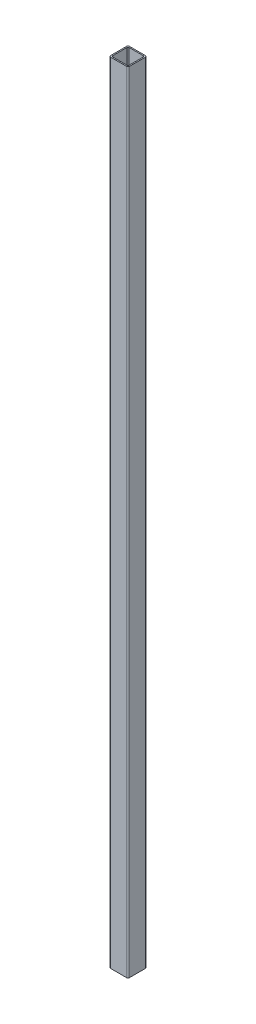
from build123d import *

# Parameters (mm, degrees)
BOSS_EXTRUDE1_DEPTH = 2100


with BuildPart() as part:
    # Sketch2 → Boss-Extrude1 (new, symmetric)
    with BuildSketch(Plane(origin=(0, 0, 0), x_dir=(1, 0, 0), z_dir=(0, 1, 0))):
        with BuildLine():
            Line((7.875, -1.525), (92.125, -1.525))
            ThreePointArc((92.125, -1.525), (97.693465902, 0.781534098), (100, 6.35))
            Line((100, 6.35), (100, 90.6))
            ThreePointArc((100, 90.6), (97.693465902, 96.168465902), (92.125, 98.475))
            Line((92.125, 98.475), (7.875, 98.475))
            ThreePointArc((7.875, 98.475), (2.306534098, 96.168465902), (0, 90.6))
            Line((0, 90.6), (0, 6.35))
            ThreePointArc((0, 6.35), (2.306534098, 0.781534098), (7.875, -1.525))
        make_face()
        with BuildLine():
            Line((12.6, 4.775), (87.4, 4.775))
            ThreePointArc((87.4, 4.775), (91.854772721, 6.620227279), (93.7, 11.075))
            Line((93.7, 11.075), (93.7, 85.875))
            ThreePointArc((93.7, 85.875), (91.854772721, 90.329772721), (87.4, 92.175))
            Line((87.4, 92.175), (12.6, 92.175))
            ThreePointArc((12.6, 92.175), (8.145227279, 90.329772721), (6.3, 85.875))
            Line((6.3, 85.875), (6.3, 11.075))
            ThreePointArc((6.3, 11.075), (8.145227279, 6.620227279), (12.6, 4.775))
        make_face(mode=Mode.SUBTRACT)
    extrude(amount=BOSS_EXTRUDE1_DEPTH, both=True)


solid = part.part
